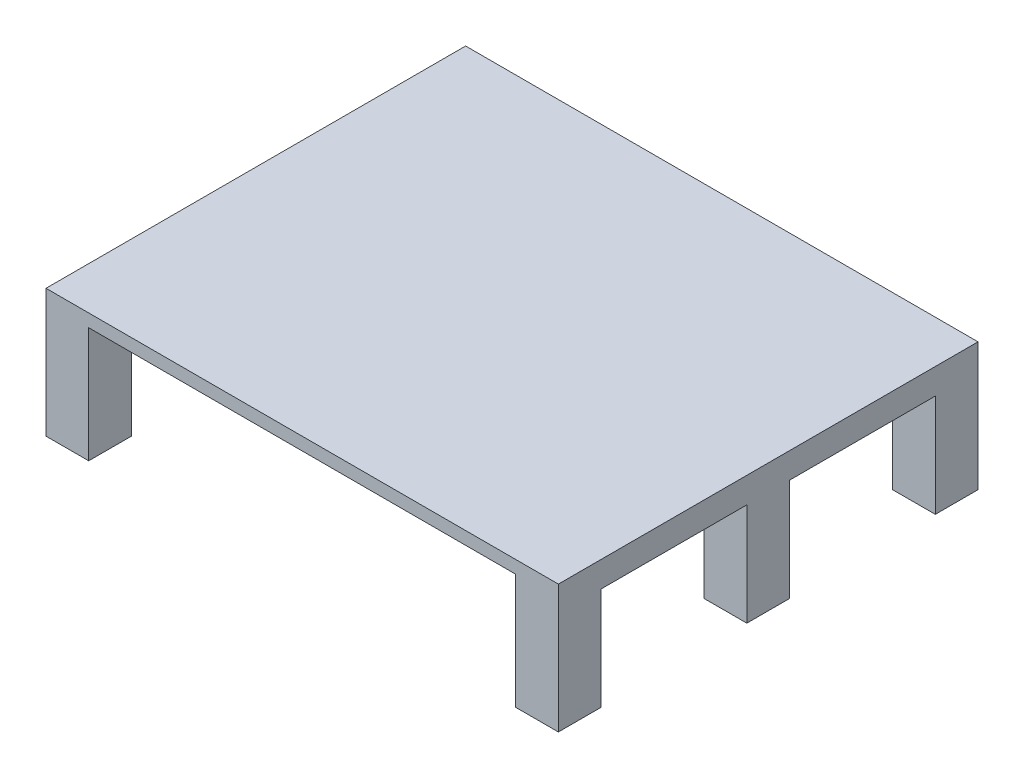
from build123d import *

# Parameters (mm, degrees)
BOSS_EXTRUDE1_DEPTH      = 435
BOSS_EXTRUDE1_DEPTH_BACK = 4479
SKETCH3_W                = 1707
SKETCH3_H                = 1200
CUT_EXTRUDE1_DEPTH       = 7637.192834129


with BuildPart() as part:
    # Sketch2 → Boss-Extrude1 (new, two sides: drawn at the far end of the back side and taken through both)
    with BuildSketch(Plane.XY.offset(-BOSS_EXTRUDE1_DEPTH_BACK)):
        Polygon((3000, -1500), (2500, -1500), (2500, -150), (-2500, -150), (-2500, -1500), (-3000, -1500), (-3000, 0), (3000, 0), align=None)
    extrude(amount=BOSS_EXTRUDE1_DEPTH + BOSS_EXTRUDE1_DEPTH_BACK)

    # Sketch3 → Cut-Extrude1 (cut, through all)
    with BuildSketch(Plane(origin=(3000, 0, 0), x_dir=(0, 0, -1), z_dir=(1, 0, 0))):
        with Locations((918.5, -900)):
            Rectangle(SKETCH3_W, SKETCH3_H)
        with Locations((3125.5, -900)):
            Rectangle(SKETCH3_W, SKETCH3_H)
    extrude(amount=-CUT_EXTRUDE1_DEPTH, mode=Mode.SUBTRACT)


solid = part.part
